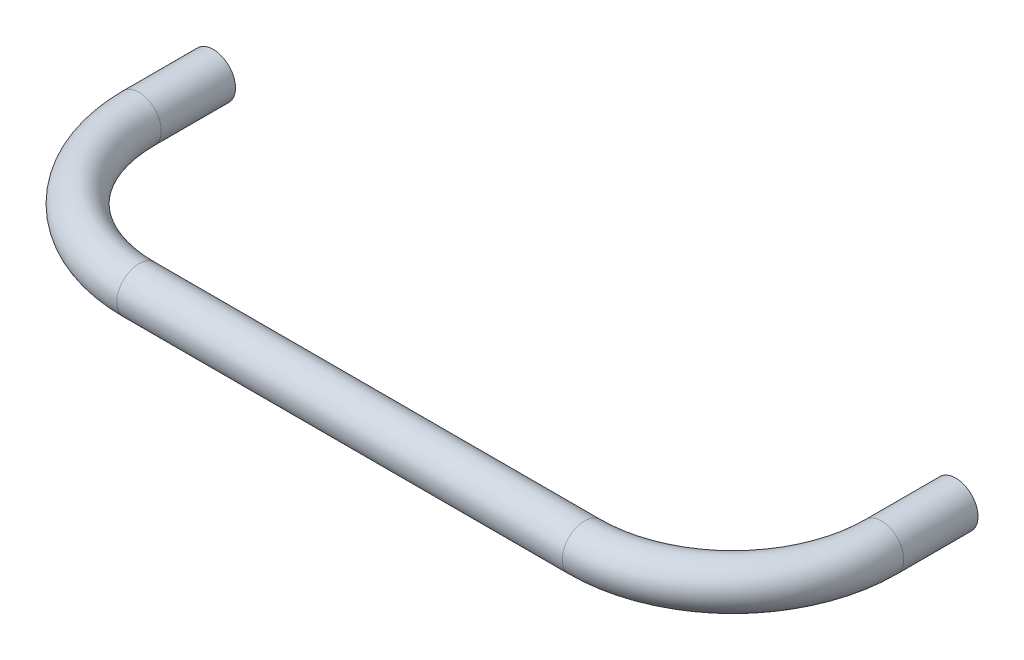
from build123d import *

# Parameters (mm, degrees)
SWEEP1_PROFILE_R       = 15
M10_TAPPED_HOLE1_D     = 8.5
M10_TAPPED_HOLE1_DEPTH = 31.5
M10_TAPPED_HOLE1_TIP   = 2.553657631


with BuildPart() as part:
    # Sweep1: sweep along a path in Sketch1
    with BuildLine(Plane(origin=(0, 0, 0), x_dir=(1, 0, 0), z_dir=(0, 1, 0))) as sweep1_path:
        Line((500, 150), (500, 100))
        ThreePointArc((500, 100), (470.710678119, 29.289321881), (400, 0))
        Line((400, 0), (100, 0))
        ThreePointArc((100, 0), (29.289321881, 29.289321881), (0, 100))
        Line((0, 100), (0, 150))
    # Sweep1 profile (on start of the path) → Sweep1 (sweep)
    with BuildSketch(Plane(origin=(500, 0, -150), x_dir=(1, 0, 0), z_dir=(0, 0, 1))):
        Circle(SWEEP1_PROFILE_R)
    sweep(path=sweep1_path.line)

    # M10 Tapped Hole1
    with Locations(Plane(origin=(0, 0, -150), x_dir=(-1, 0, 0), z_dir=(0, 0, -1))):
        with Locations((-500, 0), (0, 0)):
            Hole(M10_TAPPED_HOLE1_D / 2, depth=M10_TAPPED_HOLE1_DEPTH)
            with Locations((0, 0, -(M10_TAPPED_HOLE1_DEPTH + M10_TAPPED_HOLE1_TIP / 2))):  # 118° drill point
                Cone(0, M10_TAPPED_HOLE1_D / 2, M10_TAPPED_HOLE1_TIP, mode=Mode.SUBTRACT)


solid = part.part
